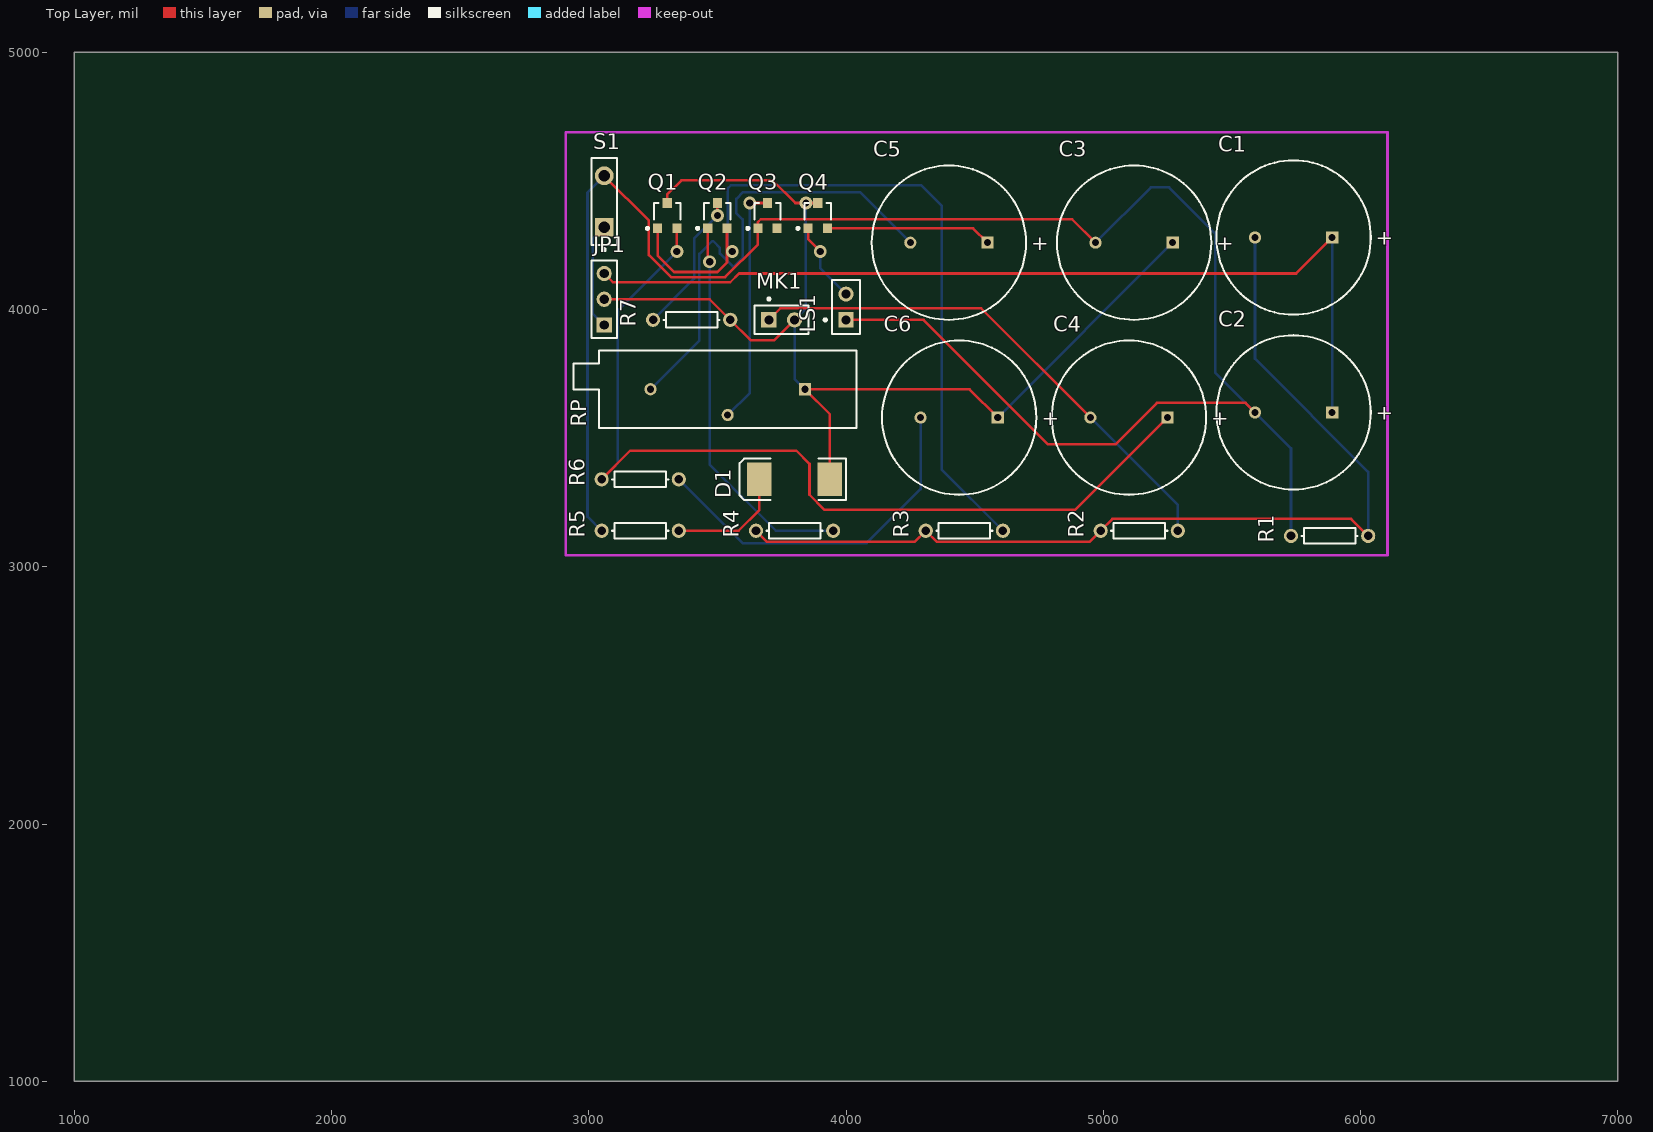
[diagram p0: Top Layer view]
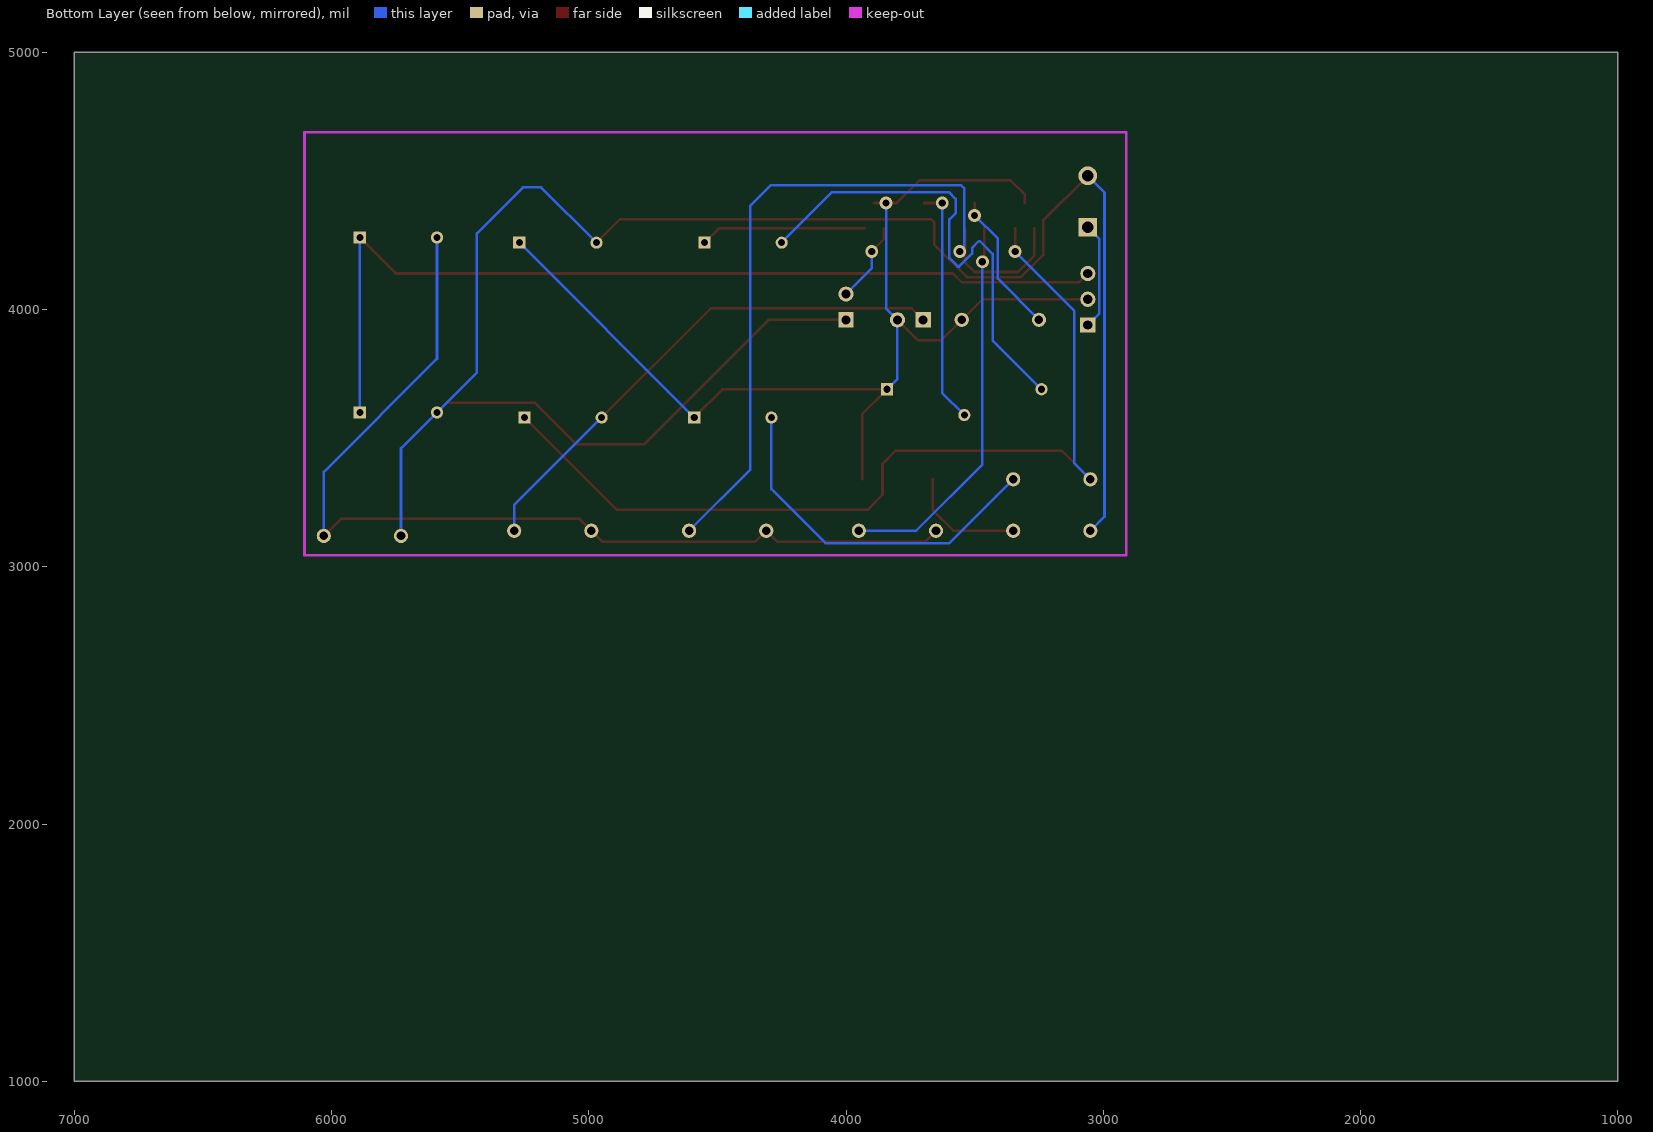
[diagram p1: Bottom Layer view, seen from below]
# Altium PCB MISC95146-6.PCBDOC
Units mil, origin at the board's own origin, x right, y up, seen from the top; angles counter-clockwise.
Board outline 6000 x 4000 mil, 2 copper layers (Top Layer, Bottom Layer); 23 components, 16 nets, 52 pads, 7 vias.

## Layer stack, top to bottom (the 12.6 mil dielectric is the usual default, probably not edited)
Top Layer: signal copper 1.4
Dielectric: dielectric 12.6, FR-4, Dk 4.8
Bottom Layer: signal copper 1.4

## Board outline
1000,1000 7000,1000 7000,5000 1000,5000

## Design rules (kind name [scope] priority, off if disabled: settings)
Clearance [All] p1: gap=10
ComponentClearance [All] p1: gap=10 collisioncheckmode=0
PolygonConnect [All] p1: connectstyle=Relief reliefconductorwidth=10 reliefentries=4 polygonreliefangle="90 Angle"
RoutingLayers [All] p1: top layer=Horizontal bottom layer=Vertical
RoutingVias [All] p1: holewidth=28 width=50 viastyle="Through Hole" minholewidth=28 minwidth=50 maxholewidth=28 maxwidth=50
SolderMaskExpansion [All] p1: expansion=4
TestPointUsage [All] p1: valid=0 allowmultiple=FALSE
Testpoint [All] p1: side=15 testpointundercomponent=TRUE minsize=40 maxsize=100 preferedsize=60 minholesize=0 maxholesize=40 preferedholesize=32 testpointgrid=1 style=1023 order=1234567890
Width [All] p1: maxlimit=10 minlimit=10 preferedwidth=10
16 further rules are at their usual default settings.

## Components (designator, comment, footprint, x,y, rotation, side; value= is the part's Value field where it differs from the comment)
C1 "Cap Pol1" RB7.6-15 5740,4280 r0 top
C2 "Cap Pol1" RB7.6-15 5740,3600 r0 top
C3 "Cap Pol1" RB7.6-15 5120,4260 r0 top
C4 "Cap Pol1" RB7.6-15 5100,3580 r0 top
C5 "Cap Pol1" RB7.6-15 4400,4260 r0 top
C6 "Cap Pol1" RB7.6-15 4440,3580 r0 top
D1 "Diode" DSO-C2/X3.3 3800,3340 r180 top
JP1 "Header 3" HDR1X3 3060,3940 r90 top
LS1 "Speaker" PIN2 4000,3960 r90 top
MK1 "Mic1" PIN2 3700,3960 r0 top
Q1 "PNP" SO-G3/C2.5 3305,4365 r0 top
Q2 "PNP" SO-G3/C2.5 3500,4365 r0 top
Q3 "PNP" SO-G3/C2.5 3695,4365 r0 top
Q4 "PNP" SO-G3/C2.5 3890,4365 r0 top
R1 "Res1" AXIAL-0.3 5880,3120 r180 top
R2 "Res1" AXIAL-0.3 5140,3140 r180 top
R3 "Res1" AXIAL-0.3 4460,3140 r180 top
R4 "Res1" AXIAL-0.3 3800,3140 r180 top
R5 "Res1" AXIAL-0.3 3200,3140 r180 top
R6 "Res1" AXIAL-0.3 3200,3340 r180 top
R7 "Res1" AXIAL-0.3 3400,3960 r180 top
RP "RPot" VR2 3540,3640 r180 top
S1 "SW-SPST" SPST-2 3060,4420 r90 top

## Footprints (in the part's own frame and the unit in brackets; to place one, negate y for a bottom-side part, rotate by r counter-clockwise, add the part's x,y. Pads: shape width x height; smd on the part's side, far side on the other; paste and mask are expansions set on the pad)
AXIAL-0.3 [mm]
  round 1.4 hole 0.85: 1(-3.81,0) 2(3.81,0)
  silkscreen extent -2.77,-0.76 2.77,0.76
DSO-C2/X3.3 [mm]
  rect 2.4x3.3 smd: 1(-3.475,0) 2(3.475,0)
  silkscreen extent -5.08,-2.05 5.42,2.06
HDR1X3 [mm] "Connector; Header; 3 Position"
  rect 1.5x1.5 hole 0.9: 1(0,0)
  round 1.5 hole 0.9: 2(2.54,0) 3(5.08,0)
  silkscreen extent -1.27,-1.27 6.35,1.27
PIN2 [mm]
  rect 1.5x1.5 hole 0.9: 1(0,0)
  round 1.5 hole 0.9: 2(2.54,0)
  silkscreen extent -1.4,-1.4 3.94,2.17
RB7.6-15 [mm]
  rect 1.2x1.2 hole 0.7: 1(3.81,0)
  round 1.2 hole 0.7: 2(-3.81,0)
  silkscreen extent -7.62,-7.62 7.62,7.62
SO-G3/C2.5 [mm]
  rect 0.9x0.95 smd: 1(-0.95,-1.25) 2(0.95,-1.25) 3(0,1.25)
  silkscreen extent -2.07,-1.37 1.3,1.25
SPST-2 [mm]
  rect 1.85x1.85 hole 1.1: 1(-2.54,0)
  round 1.85 hole 1.1: 2(2.54,0)
  silkscreen extent -4.89,-1.27 4.28,1.27
VR2 [mm]
  rect 1.2x1.2 hole 0.7: 1(-7.62,-1.27)
  round 1.2 hole 0.7: 2(0,1.27) 3(7.62,-1.27)
  silkscreen extent -12.7,-5.08 15.24,2.54

## Part data
C1 C2 C3 C4 C5 C6: "Polarized Capacitor (Radial)"
D1: "Default Diode"
JP1: "Header, 3-Pin"
LS1: "Loudspeaker"
MK1: "Microphone"
Q1 Q2 Q3 Q4: "PNP Bipolar Transistor"
R1 R2 R3 R4 R5 R6 R7: "Resistor"
RP: "Potentiometer"
S1: "Single-Pole, Single-Throw Switch"

## Via types
v1: diameter 50, hole 28, Top Layer to Bottom Layer, 7 vias

## Nets (pads, with @x,y where several pads share a name; then routed paths per layer and width w, separated by ;. In a path a pad name is that pad's centre, name@x,y a point inside that pad or via, vN(x,y) a via of type N, cw(c..) or ccw(c..) an arc to the next point about the centre after c; other vN are vias at no path point)
GND: C1.1 C2.1 JP1.3 | length 3596.2
  Top Layer w10: JP1.3 3094,4106 3550,4106 3584,4140 5750,4140 C1.1
  Bottom Layer w10: C2.1 C1.1
NetC1_2: C1.2 R1.1 R2.2 R3.2 R4.2 | length 3839.9
  Top Layer w10: R4.2 3693,3097 4267,3097 R3.2 4353,3097 4947,3097 R2.2 5036,3186 5964,3186 R1.1
  Bottom Layer w10: C1.2 5590,3809 6030,3369 R1.1
NetC2_2: C2.2 C3.2 LS1.1 Q3.1 R1.2 R5.2 S1.2 | length 7561.8
  Top Layer w10: S1.2 3234,4346 3234,4212 3320,4126 3530,4126 3657.6,4253.6 Q3.1 3657.6,4340 3668.6,4351 4879,4351 C3.2 ; LS1.1 4302,3960 4786,3476 5048,3476 5209,3637 5553,3637 C2.2
  Bottom Layer w10: R5.2 2995,3195 2995,4455 S1.2 ; C3.2 5185,4475 5256,4475 5435,4296 5435,3755 C2.2 5730,3460 R1.2
NetC3_1: C3.1 C6.1 D1.1 JP1.2 MK1.2 Q1.3 Q4.3 R7.1 RP.1 | length 4422.7
  Top Layer w10: JP1.2 3470,4040 R7.1 3630,3880 3720,3880 MK1.2 ; Q1.3 3305,4447 3360,4502 3715.21,4502 3803,4414.21 v1(3844,4414.21) Q4.3 ; D1.1 3936.81,3593.19 RP.1 4480,3690 C6.1
  Bottom Layer w10: RP.1 3800,3730 MK1.2 3844,4004 v1(3844,4414.21) ; C6.1 C3.1
NetC4_1: C4.1 Q1.2 R6.2 | length 3657.1
  Top Layer w10: R6.2 3161,3451 3807,3451 3858,3400 3858,3280 3917,3221 4891,3221 C4.1 ; v1(3342.4,4225.4) Q1.2
  Bottom Layer w10: R6.2 3113,3403 3113,3996 v1(3342.4,4225.4)
NetC4_2: C4.2 MK1.1 R2.1 | length 2025.5
  Top Layer w10: MK1.1 3745,4005 4525,4005 C4.2
  Bottom Layer w10: C4.2 5290,3240 R2.1
NetC5_1: C5.1 Q4.2 | length 645.7
  Top Layer w10: Q4.2 4494.21,4315.79 C5.1
NetC5_2: C5.2 RP.3 | length 1869.5
  Bottom Layer w10: RP.3 3430,3880 3430,4216 3480,4266 3484,4266 3510,4240 3510,4217 3560,4167 3565,4167 3598,4200 3598,4350 3574,4374 3574,4430 3600,4456 4054,4456 C5.2
NetC6_2: C6.2 R6.1 | length 1407.7
  Bottom Layer w10: R6.1 3598,3092 4080,3092 4290,3302 C6.2
NetD1_2: D1.2 R5.1 | length 465.6
  Top Layer w10: R5.1 3582,3140 3663.19,3221.19 D1.2
NetJP1_1: JP1.1 S1.1 | length 417.3
  Bottom Layer w10: JP1.1 3015,3985 3015,4275 S1.1
NetLS1_2: LS1.2 Q4.1 | length 316.8
  Top Layer w10: Q4.1 3852.6,4273.4 v1(3900,4226)
  Bottom Layer w10: v1(3900,4226) 3900,4160 LS1.2
NetQ1_1: Q1.1 Q2.2 R3.1 | length 3063.6
  Top Layer w10: Q1.1 3267.6,4210.4 3332,4146 3500,4146 3537.4,4183.4 3537.4,4226 3537.4,4246.6 ; Q2.2 3537.4,4246.6 ; v1(3558,4226) 3537.4,4246.6
  Bottom Layer w10: v1(3558,4226) 3540,4244 3540,4471 3552,4483 4293,4483 4372,4404 4372,3378 R3.1
NetQ2_1: Q2.1 R4.1 | length 1507.7
  Top Layer w10: Q2.1 3462.6,4193.4 v1(3470,4186)
  Bottom Layer w10: v1(3470,4186) 3470,3398 3728,3140 R4.1
NetQ2_3: Q2.3 R7.2 | length 557.8
  Top Layer w10: v1(3500,4366) Q2.3
  Bottom Layer w10: R7.2 3410,4120 3410,4276 v1(3500,4366)
NetQ3_3: Q3.3 RP.2 | length 928.8
  Top Layer w10: v1(3626,4414.21) Q3.3
  Bottom Layer w10: RP.2 3626,3676 v1(3626,4414.21)
pads on no net: Q3.2

## Keep-outs
Keep-Out Layer:
  lines w10: 2910,3045 6105,3045 6105,4690 2910,4690 2910,3045